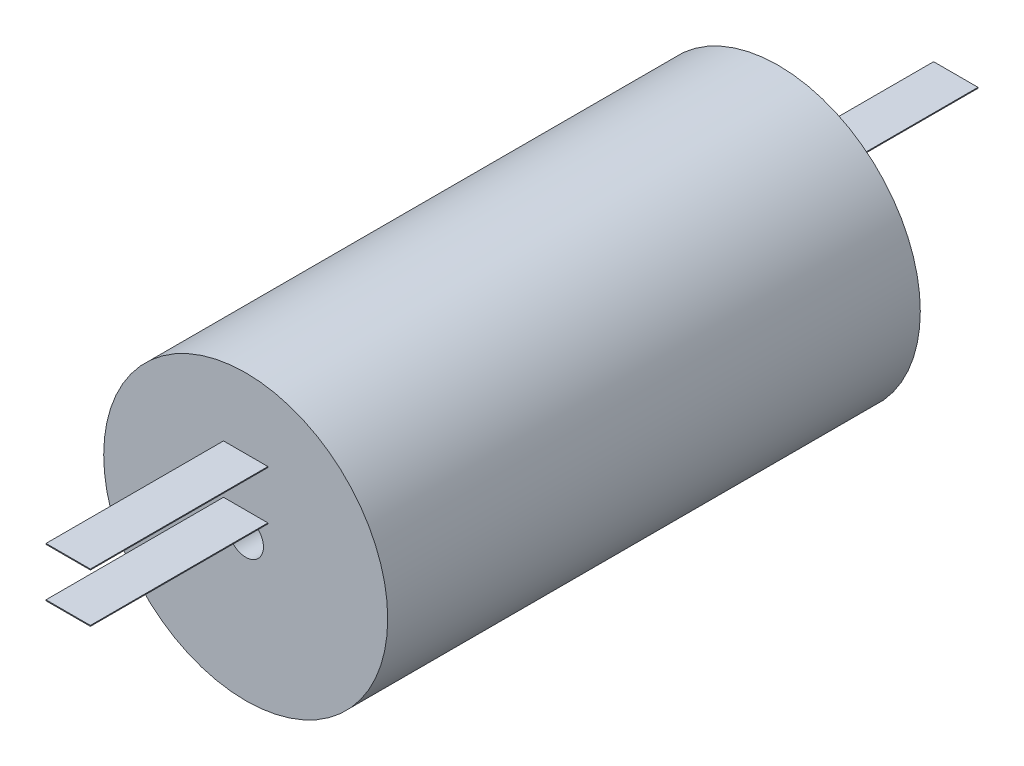
from build123d import *

# Parameters (mm, degrees)
SKETCH1_R           = 16
SKETCH1_R_2         = 2
BOSS_EXTRUDE1_DEPTH = 60
SKETCH2_W           = 5
SKETCH2_H           = 0.1
BOSS_EXTRUDE2_DEPTH = 20
SKETCH3_W           = 5
SKETCH3_H           = 0.1
BOSS_EXTRUDE3_DEPTH = 20


with BuildPart() as part:
    # Sketch1 → Boss-Extrude1 (new body)
    with BuildSketch(Plane.XY):
        Circle(SKETCH1_R)
        Circle(SKETCH1_R_2, mode=Mode.SUBTRACT)
    extrude(amount=BOSS_EXTRUDE1_DEPTH)

    # Sketch2 → Boss-Extrude2 (add)
    with BuildSketch(Plane(origin=(0, 0, 0), x_dir=(-1, 0, 0), z_dir=(0, 0, -1))):
        with Locations((0, 5.05)):
            Rectangle(SKETCH2_W, SKETCH2_H)
    extrude(amount=BOSS_EXTRUDE2_DEPTH)

    # Sketch3 → Boss-Extrude3 (add)
    with BuildSketch(Plane.XY.offset(60)):
        with Locations((0, 8.05)):
            Rectangle(SKETCH3_W, SKETCH3_H)
        with Locations((0, 2.55)):
            Rectangle(SKETCH3_W, SKETCH3_H)
    extrude(amount=BOSS_EXTRUDE3_DEPTH)


solid = part.part
